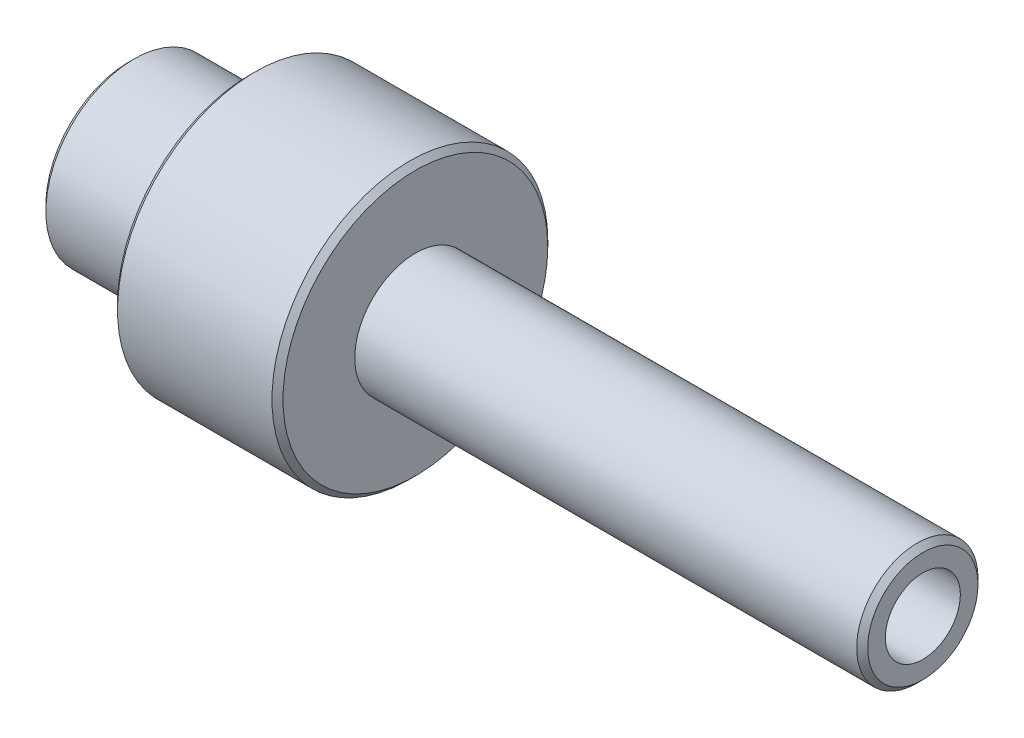
SolidWorks part; units mm, degrees
ref_plane "Front Plane" through (0, 0, 0) normal (0, 0, 1) x (1, 0, 0)
ref_plane "Top Plane" through (0, 0, 0) normal (0, 1, 0) x (1, 0, 0)
ref_plane "Right Plane" through (0, 0, 0) normal (1, 0, 0) x (0, 0, -1)
other "Configuration Table"
sketch "Sketch1" plane through (0, 0, 0) normal (1, 0, 0) x (0, 0, -1)
  circle A0 centre (0, 0) radius 8
  dimension "D1" = 16
extrude "Boss-Extrude1" add sketch "Sketch1" along normal blind 11
sketch "Sketch2" plane through (11, 0, 0) normal (1, 0, 0) x (0, 0, -1)
  circle A0 centre (0, 0) radius 12.5
  dimension "D1" = 25
extrude "Boss-Extrude2" add sketch "Sketch2" along normal blind 15
sketch "Sketch3" plane through (26, 0, 0) normal (1, 0, 0) x (0, 0, -1)
  circle A0 centre (0, 0) radius 5.5
  dimension "D1" = 11
extrude "Boss-Extrude3" add sketch "Sketch3" along normal blind 46
sketch "Sketch5" plane through (0, 0, 0) normal (-1, 0, 0) x (0, 0, 1)
  circle A0 centre (0, 0) radius 5.5
  dimension "D1" = 11
extrude "Cut-Extrude1" cut sketch "Sketch5" against normal blind 11
sketch "Sketch6" plane through (0, 0, 0) normal (-1, 0, 0) x (0, 0, 1)
  circle A0 centre (0, 0) radius 6
  dimension "D1" = 12
extrude "Cut-Extrude2" cut sketch "Sketch6" against normal blind 1.1 from offset 2.7 offset against normal yes
sketch "Sketch7" plane through (3.8, 0, 0) normal (-1, 0, 0) x (0, 0, 1)
  circle A0 centre (0, 0) radius 5
  dimension "D1" = 10
extrude "Cut-Extrude3" cut sketch "Sketch7" against normal blind 10.2
sketch "Sketch8" plane through (14, 0, 0) normal (-1, 0, 0) x (0, 0, 1)
  circle A0 centre (0, 0) radius 3
  dimension "D1" = 6
extrude "Cut-Extrude4" cut sketch "Sketch8" against normal blind 15
hole_wizard "M8 Tapped Hole1" positions "Sketch9" profile "Sketch10" tap size "M8" standard "GB"
sketch "Sketch9" plane through (72, 0, 0) normal (1, 0, 0) x (0, 0, -1)
  point P0 (0, 0)
sketch "Sketch10" plane through (72, 0, 0) normal (0, 1, 0) x (0, 0, -1)
  line L0 (0, 0) -> (0, 13.0429)
  line L1 (0, 13.0429) -> (3.4, 11)
  line L2 (3.4, 11) -> (3.4, 0)
  line L5 (3.4, 0) -> (0, 0)
  line L10 (0, 13.0429) -> (-3.4, 11) construction
  line L11 (0, -6.35) -> (0, 107.95) construction
  dimension "螺纹孔钻头直径" = 6.8
  dimension "螺纹孔钻头深度" = 11
  dimension "导头角度" = 118
cosmetic thread "Hole Thread Line1" parameters "D1"=11, "D2"=8
sketch "Sketch11" plane through (72, 0, 0) normal (1, 0, 0) x (0, 0, -1)
  circle A0 centre (0, 0) radius 5.5
  dimension "D1" = 11
extrude "Boss-Extrude4" add sketch "Sketch11" against normal blind 5 from offset 11 offset against normal yes
sketch "Sketch12" plane through (61, 0, 0) normal (1, 0, 0) x (0, 0, -1)
  circle A0 centre (0, 0) radius 2.75
  dimension "D1" = 5.5
extrude "Cut-Extrude5" cut sketch "Sketch12" against normal blind 5
sketch "Sketch13" plane through (56, 0, 0) normal (1, 0, 0) x (0, 0, -1)
  circle A0 centre (0, 0) radius 1.5
  dimension "D1" = 3
extrude "Cut-Extrude6" cut sketch "Sketch13" against normal blind 88
chamfer "Chamfer1" distance 0.5 angle 45 4 edges at (0, 0, -8) (72, 0, -5.5) (26, 0, -12.5) (11, 0, -12.5)
